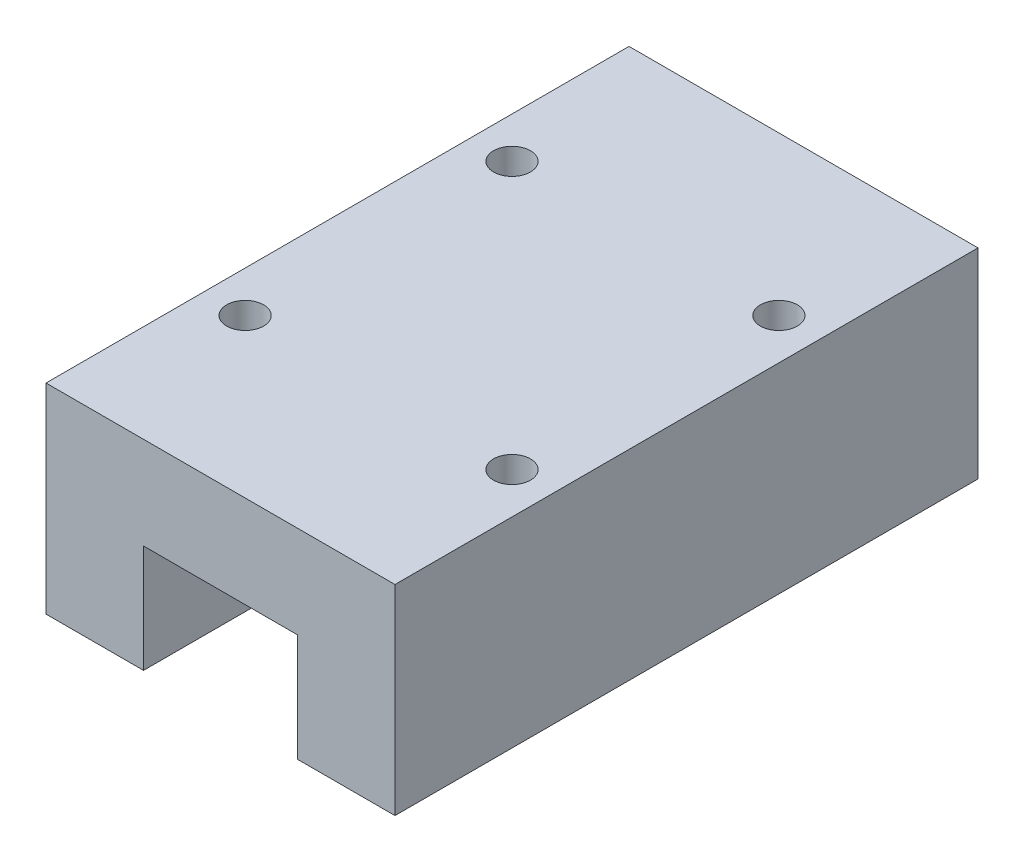
from build123d import *

# Parameters (mm, degrees)
SKETCH_1_W               = 34
SKETCH_1_H               = 19.5
EXTRUDE_1_DEPTH          = 28.4
CUT_EXTRUDE_1_DEPTH      = 35.505398128
CUT_EXTRUDE_1_DEPTH_BACK = 35.505398128
SKETCH_2_W               = 15
SKETCH_2_H               = 10.5
SKETCH_4_R               = 1.8
CUT_EXTRUDE_2_DEPTH      = 6


with BuildPart() as part:
    # 草图1 → 凸台-拉伸1 (new, symmetric)
    with BuildSketch(Plane.XY):
        Rectangle(SKETCH_1_W, SKETCH_1_H)
    extrude(amount=EXTRUDE_1_DEPTH, both=True)

    # 草图2 → 切除-拉伸1 (cut, two sides: drawn at the far end of the back side and taken through both)
    with BuildSketch(Plane.XY.offset(-CUT_EXTRUDE_1_DEPTH_BACK)):
        with Locations((0, -4.5)):
            Rectangle(SKETCH_2_W, SKETCH_2_H)
    extrude(amount=CUT_EXTRUDE_1_DEPTH + CUT_EXTRUDE_1_DEPTH_BACK, mode=Mode.SUBTRACT)

    # 草图4 → 切除-拉伸2 (cut)
    with BuildSketch(Plane(origin=(0, 9.75, 0), x_dir=(1, 0, 0), z_dir=(0, 1, 0))):
        with Locations(Location((-13, 13, 0), (0, 0, 270))):
            Circle(SKETCH_4_R)
        with Locations(Location((13, 13, 0), (0, 0, 90))):
            Circle(SKETCH_4_R)
        with Locations(Location((13, -13, 0), (0, 0, 270))):
            Circle(SKETCH_4_R)
        with Locations(Location((-13, -13, 0), (0, 0, 90))):
            Circle(SKETCH_4_R)
    extrude(amount=-CUT_EXTRUDE_2_DEPTH, mode=Mode.SUBTRACT)


solid = part.part
